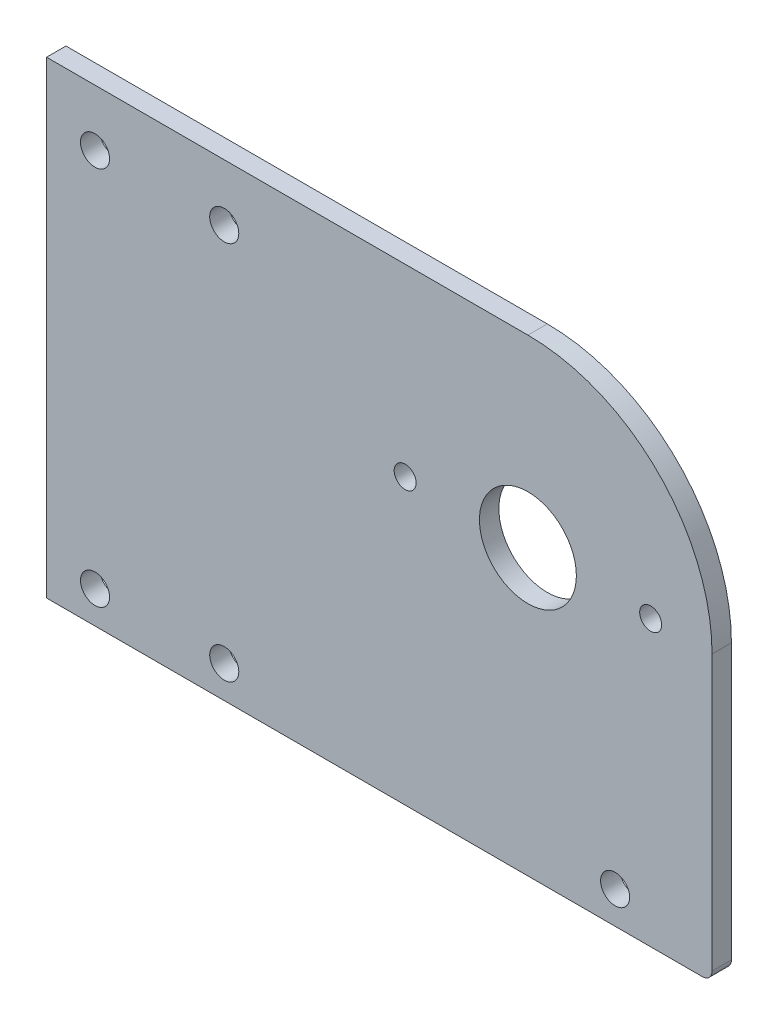
from build123d import *

# Parameters (mm, degrees)
SKETCH_1_W               = 206
SKETCH_1_H               = 145
EXTRUDE_1_DEPTH          = 6
SKETCH_3_R               = 4.5
CUT_EXTRUDE_2_DEPTH      = 127.100158604
SKETCH_4_R               = 15
CUT_EXTRUDE_3_DEPTH      = 127.100158604
FILLET_1_R               = 57
HOLE_WIZARD_M8_1_D       = 6.8
PATTERN_CIRCULAR_1_COUNT = 2
SKETCH_11_R              = 4.5
CUT_EXTRUDE_6_DEPTH      = 127.100158604
FILLET_5_R               = 3


with BuildPart() as part:
    # 草图1 → 凸台-拉伸1 (new body)
    with BuildSketch(Plane.XY):
        Rectangle(SKETCH_1_W, SKETCH_1_H)
    extrude(amount=EXTRUDE_1_DEPTH)

    # 草图3 → 切除-拉伸2 (cut, through all)
    with BuildSketch(Plane.XY.offset(6)):
        with Locations((-88, 55)):
            Circle(SKETCH_3_R)
        with Locations((-48, 55)):
            Circle(SKETCH_3_R)
        with Locations((-88, -62.5)):
            Circle(SKETCH_3_R)
        with Locations((-48, -62.5)):
            Circle(SKETCH_3_R)
    extrude(amount=-CUT_EXTRUDE_2_DEPTH, mode=Mode.SUBTRACT)

    # 草图4 → 切除-拉伸3 (cut, through all)
    with BuildSketch(Plane.XY.offset(6)):
        with Locations((46, 15.5)):
            Circle(SKETCH_4_R)
    extrude(amount=-CUT_EXTRUDE_3_DEPTH, mode=Mode.SUBTRACT)

    # 圆角1
    fillet_1_edges = [part.edges().sort_by_distance(p)[0] for p in [
        (103, 72.5, 3),
    ]]
    fillet(fillet_1_edges, radius=FILLET_1_R)

    # M8 螺纹孔1 (through all)
    with Locations(Plane.XY.offset(6)):
        with Locations((8, 15.5)):
            hole_wizard_m8_1 = Hole(HOLE_WIZARD_M8_1_D / 2)

    # 阵列(圆周)1: M8 螺纹孔1 ×2 about axis
    pattern_circular_1_axis = Axis((46, 15.5, 0), (0, 0, 1))
    for i in range(1, PATTERN_CIRCULAR_1_COUNT):
        add(hole_wizard_m8_1.rotate(pattern_circular_1_axis, i * 360 / PATTERN_CIRCULAR_1_COUNT), mode=Mode.SUBTRACT)

    # 草图11 → 切除-拉伸6 (cut, through all)
    with BuildSketch(Plane.XY.offset(6)):
        with Locations((73, -62.5)):
            Circle(SKETCH_11_R)
    extrude(amount=-CUT_EXTRUDE_6_DEPTH, mode=Mode.SUBTRACT)

    # 圆角5
    fillet_5_edges = [part.edges().sort_by_distance(p)[0] for p in [
        (103, -72.5, 3),
    ]]
    fillet(fillet_5_edges, radius=FILLET_5_R)


solid = part.part
